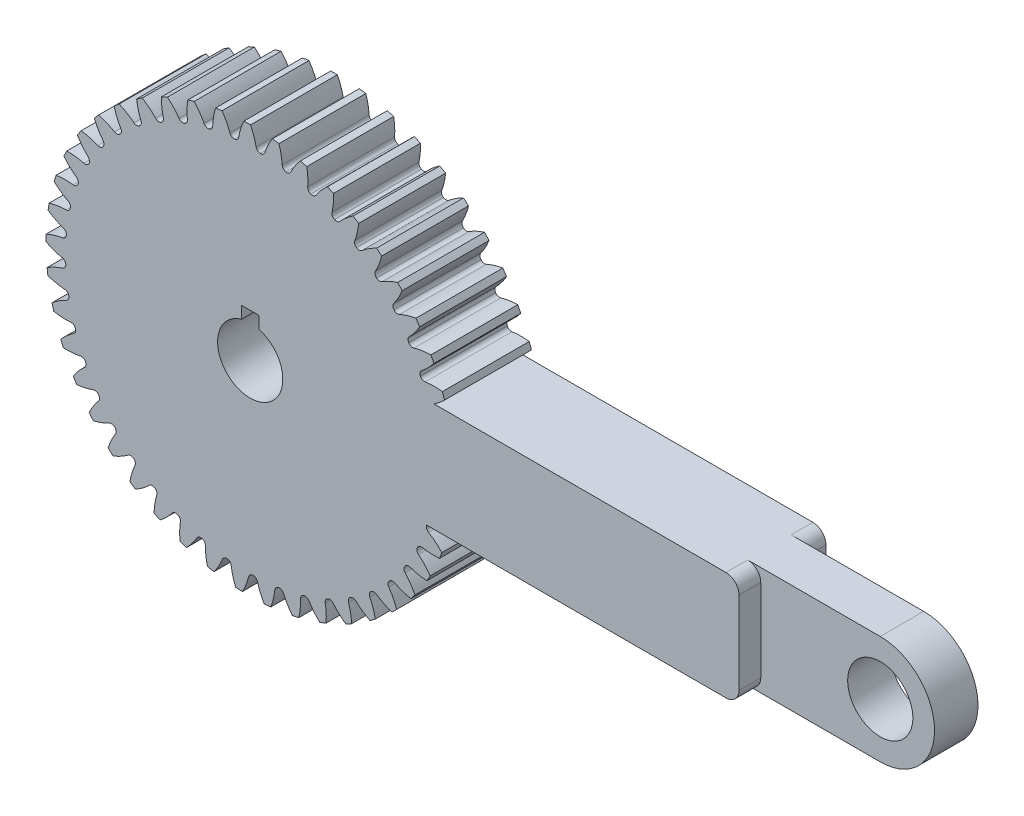
from build123d import *

# Parameters (mm, degrees)
SKETCH1_R           = 7.5
BOSS_EXTRUDE1_DEPTH = 20
SKETCH2_W           = 40
SKETCH2_H           = 7.746884482
SKETCH2_H_2         = 5
CUT_EXTRUDE1_DEPTH  = 41
FILLET1_R           = 3
SCALE1_SCALE        = 0.3


with BuildPart() as part:
    # Sketch1 → Boss-Extrude1 (new body)
    with BuildSketch(Plane(origin=(0, 0, 0), x_dir=(-1, 0, 0), z_dir=(0, 0, -1))):
        with BuildLine():
            Line((-140, -12.5), (-40.620192023, -12.5))
            ThreePointArc((-40.620192023, -12.5), (-40.610112054, -12.532709162), (-40.600005747, -12.565410195))
            ThreePointArc((-40.600005747, -12.565410195), (-40.621924881, -13.219969243), (-41.044194735, -13.720585031))
            ThreePointArc((-41.044194735, -13.720585031), (-42.659259377, -14.876128654), (-44.106676084, -16.235797635))
            ThreePointArc((-44.106676084, -16.235797635), (-43.835198922, -16.955097625), (-43.551992177, -17.669860707))
            ThreePointArc((-43.551992177, -17.669860707), (-41.566460224, -17.699832016), (-39.594088642, -17.469645664))
            ThreePointArc((-39.594088642, -17.469645664), (-38.94485587, -17.555812971), (-38.488181859, -18.025256092))
            ThreePointArc((-38.488181859, -18.025256092), (-38.472167175, -18.059411753), (-38.45612218, -18.093553185))
            ThreePointArc((-38.45612218, -18.093553185), (-38.386730986, -18.744792664), (-38.735219087, -19.299305098))
            ThreePointArc((-38.735219087, -19.299305098), (-40.173745442, -20.668376604), (-41.417846641, -22.216254852))
            ThreePointArc((-41.417846641, -22.216254852), (-41.048904266, -22.890772346), (-40.668977875, -23.559164642))
            ThreePointArc((-40.668977875, -23.559164642), (-38.698597783, -23.312511632), (-36.777456933, -22.81006437))
            ThreePointArc((-36.777456933, -22.81006437), (-36.122550279, -22.805037364), (-35.604986733, -23.206355158))
            ThreePointArc((-35.604986733, -23.206355158), (-35.584374354, -23.237949606), (-35.563733938, -23.269525744))
            ThreePointArc((-35.563733938, -23.269525744), (-35.404383037, -23.904770017), (-35.672306461, -24.502386144))
            ThreePointArc((-35.672306461, -24.502386144), (-36.906295249, -26.058338114), (-37.922865925, -27.764297939))
            ThreePointArc((-37.922865925, -27.764297939), (-37.463639381, -28.38090422), (-36.994388179, -28.989916235))
            ThreePointArc((-36.994388179, -28.989916235), (-35.077511154, -28.471439728), (-33.244993859, -27.706511118))
            ThreePointArc((-33.244993859, -27.706511118), (-32.597160335, -27.610387645), (-32.02878104, -27.935768919))
            ThreePointArc((-32.02878104, -27.935768919), (-32.003972162, -27.964187202), (-31.979138069, -27.992583453))
            ThreePointArc((-31.979138069, -27.992583453), (-31.732929044, -28.599468214), (-31.915072966, -29.228556115))
            ThreePointArc((-31.915072966, -29.228556115), (-32.920506, -30.941103714), (-33.68975976, -32.771940549))
            ThreePointArc((-33.68975976, -32.771940549), (-33.149187369, -33.318634077), (-32.599744797, -33.856412084))
            ThreePointArc((-32.599744797, -33.856412084), (-30.773680671, -33.076203635), (-29.065454795, -32.063682143))
            ThreePointArc((-29.065454795, -32.063682143), (-28.437303745, -31.878333137), (-27.829171557, -32.121444713))
            ThreePointArc((-27.829171557, -32.121444713), (-27.800649056, -32.146133703), (-27.772104652, -32.170797366))
            ThreePointArc((-27.772104652, -32.170797366), (-27.443829683, -32.737510293), (-27.536648879, -33.385825488))
            ThreePointArc((-27.536648879, -33.385825488), (-28.293956547, -35.221635925), (-28.800920743, -37.141714612))
            ThreePointArc((-28.800920743, -37.141714612), (-28.189524132, -37.607854621), (-27.570584464, -38.063931383))
            ThreePointArc((-27.570584464, -38.063931383), (-25.870875498, -37.037176862), (-24.320189715, -35.796770067))
            ThreePointArc((-24.320189715, -35.796770067), (-23.723947383, -35.525803135), (-23.087898904, -35.681913124))
            ThreePointArc((-23.087898904, -35.681913124), (-23.056217939, -35.702392278), (-23.024518809, -35.722843303))
            ThreePointArc((-23.024518809, -35.722843303), (-22.620567394, -36.238353972), (-22.622255243, -36.893277744))
            ThreePointArc((-22.622255243, -36.893277744), (-23.116697415, -38.816619056), (-23.351504565, -40.788567449))
            ThreePointArc((-23.351504565, -40.788567449), (-22.681183873, -41.165081053), (-22.004794066, -41.530579554))
            ThreePointArc((-22.004794066, -41.530579554), (-20.464523162, -40.27726357), (-19.101559806, -38.83311458))
            ThreePointArc((-19.101559806, -38.83311458), (-18.548831372, -38.481803785), (-17.897246562, -38.547873684))
            ThreePointArc((-17.897246562, -38.547873684), (-17.863023766, -38.563744397), (-17.828786897, -38.579584728))
            ThreePointArc((-17.828786897, -38.579584728), (-17.357021491, -39.033859312), (-17.267545142, -39.682644314))
            ThreePointArc((-17.267545142, -39.682644314), (-17.489498062, -41.656080851), (-17.447577912, -43.641517217))
            ThreePointArc((-17.447577912, -43.641517217), (-16.731380169, -43.921076007), (-16.010705382, -44.188882235))
            ThreePointArc((-16.010705382, -44.188882235), (-14.65985216, -42.733399158), (-13.511139763, -41.11361669))
            ThreePointArc((-13.511139763, -41.11361669), (-13.012683457, -40.688799898), (-12.358244672, -40.663543729))
            ThreePointArc((-12.358244672, -40.663543729), (-12.322146155, -40.674497098), (-12.286037928, -40.68541842))
            ThreePointArc((-12.286037928, -40.68541842), (-11.755640908, -41.069614981), (-11.576741916, -41.699633351))
            ThreePointArc((-11.576741916, -41.699633351), (-11.521885523, -43.684754415), (-11.204054002, -45.645034494))
            ThreePointArc((-11.204054002, -45.645034494), (-10.455919182, -45.822197176), (-9.704986529, -45.987098587))
            ThreePointArc((-9.704986529, -45.987098587), (-8.569843811, -44.35777774), (-7.657740753, -42.593889017))
            ThreePointArc((-7.657740753, -42.593889017), (-7.22325846, -42.103834802), (-6.578703608, -41.98774415))
            ThreePointArc((-6.578703608, -41.98774415), (-6.541431984, -41.993566979), (-6.504155206, -41.999356722))
            ThreePointArc((-6.504155206, -41.999356722), (-5.925450147, -42.30599731), (-5.660610577, -42.904986457))
            ThreePointArc((-5.660610577, -42.904986457), (-5.330012588, -44.863153925), (-4.742455924, -46.760123094))
            ThreePointArc((-4.742455924, -46.760123094), (-3.976945621, -46.831441399), (-3.210371153, -46.890228375))
            ThreePointArc((-3.210371153, -46.890228375), (-2.3130332, -45.118782634), (-1.65529253, -43.245119744))
            ThreePointArc((-1.65529253, -43.245119744), (-1.293240953, -42.699366455), (-0.671115561, -42.494700892))
            ThreePointArc((-0.671115561, -42.494700892), (-0.633396281, -42.495279846), (-0.595676502, -42.495825319))
            ThreePointArc((-0.595676502, -42.495825319), (0.020072761, -42.718941524), (0.365698108, -43.275242806))
            ThreePointArc((0.365698108, -43.275242806), (0.965602978, -45.168343175), (1.811448663, -46.965079088))
            ThreePointArc((1.811448663, -46.965079088), (2.579434662, -46.929164885), (3.346730446, -46.880693204))
            ThreePointArc((3.346730446, -46.880693204), (3.98879797, -45.001601746), (4.379374079, -43.054633405))
            ThreePointArc((4.379374079, -43.054633405), (4.661948018, -42.46380351), (5.249534987, -42.174546618))
            ThreePointArc((5.249534987, -42.174546618), (5.28696776, -42.169870428), (5.324396368, -42.165161014))
            ThreePointArc((5.324396368, -42.165161014), (5.965204976, -42.300410133), (6.384888895, -42.803195778))
            ThreePointArc((6.384888895, -42.803195778), (7.242424181, -44.594382004), (8.330095463, -46.255913239))
            ThreePointArc((8.330095463, -46.255913239), (9.085609184, -46.113465558), (9.838691744, -45.958678666))
            ThreePointArc((9.838691744, -45.958678666), (10.212991726, -44.008515868), (10.328801154, -42.026137602))
            ThreePointArc((10.328801154, -42.026137602), (10.526397473, -41.401730931), (11.068009308, -41.033512767))
            ThreePointArc((11.068009308, -41.033512767), (11.104426988, -41.02367245), (11.14083592, -41.013799812))
            ThreePointArc((11.14083592, -41.013799812), (11.794231262, -41.058549375), (12.279805082, -41.498033232))
            ThreePointArc((12.279805082, -41.498033232), (13.378279836, -43.152441912), (14.68660643, -44.646428654))
            ThreePointArc((14.68660643, -44.646428654), (15.414942657, -44.400220077), (16.139154098, -44.142130726))
            ThreePointArc((16.139154098, -44.142130726), (16.238401215, -42.158854289), (16.077189862, -40.179650834))
            ThreePointArc((16.077189862, -40.179650834), (16.185962575, -39.533820753), (16.671057417, -39.093808264))
            ThreePointArc((16.671057417, -39.093808264), (16.705751176, -39.078995351), (16.740431772, -39.064151649))
            ThreePointArc((16.740431772, -39.064151649), (17.393696251, -39.017530657), (17.935708832, -39.385158673))
            ThreePointArc((17.935708832, -39.385158673), (19.253742491, -40.870588623), (20.757259308, -42.16795212))
            ThreePointArc((20.757259308, -42.16795212), (21.444241806, -41.822774816), (22.125486176, -41.466406421))
            ThreePointArc((22.125486176, -41.466406421), (21.947748694, -39.488618565), (21.512654358, -37.551112866))
            ThreePointArc((21.512654358, -37.551112866), (21.530486327, -36.896429724), (21.949622357, -36.393187253))
            ThreePointArc((21.949622357, -36.393187253), (21.981916919, -36.37369006), (22.014194163, -36.35416421))
            ThreePointArc((22.014194163, -36.35416421), (22.654612728, -36.217080086), (23.242514411, -36.5056968))
            ThreePointArc((23.242514411, -36.5056968), (24.754452949, -37.793235816), (26.423895745, -38.868724364))
            ThreePointArc((26.423895745, -38.868724364), (27.056153181, -38.431296817), (27.681170833, -37.983585683))
            ThreePointArc((27.681170833, -37.983585683), (27.229908211, -36.049781799), (26.529399506, -34.1916852))
            ThreePointArc((26.529399506, -34.1916852), (26.455943653, -33.540891659), (26.800962865, -32.984214248))
            ThreePointArc((26.800962865, -32.984214248), (26.830229654, -32.960412266), (26.859475304, -32.936584316))
            ThreePointArc((26.859475304, -32.936584316), (27.474582938, -32.711705248), (28.096930885, -32.915693064))
            ThreePointArc((28.096930885, -32.915693064), (29.773346139, -33.980280664), (31.576221108, -34.8129611))
            ThreePointArc((31.576221108, -34.8129611), (32.14144731, -34.29179734), (32.698072986, -33.761457655))
            ThreePointArc((32.698072986, -33.761457655), (31.982068538, -31.909277036), (31.029780071, -30.166755274))
            ThreePointArc((31.029780071, -30.166755274), (30.866466129, -29.53251829), (31.130653116, -28.933241031))
            ThreePointArc((31.130653116, -28.933241031), (31.156322487, -28.905597539), (31.181967311, -28.877931273))
            ThreePointArc((31.181967311, -28.877931273), (31.759791642, -28.569634276), (32.404472559, -28.685022803))
            ThreePointArc((32.404472559, -28.685022803), (34.212735012, -29.505938), (36.113951245, -30.079603147))
            ThreePointArc((36.113951245, -30.079603147), (36.601144728, -29.484847034), (37.078544342, -28.882201257))
            ThreePointArc((37.078544342, -28.882201257), (36.11173428, -27.147694492), (34.926201261, -25.554663771))
            ThreePointArc((34.926201261, -25.554663771), (34.676207952, -24.949328045), (34.854420615, -24.31911519))
            ThreePointArc((34.854420615, -24.31911519), (34.875992943, -24.288168236), (34.897537793, -24.257202146))
            ThreePointArc((34.897537793, -24.257202146), (35.426832129, -23.871487871), (36.081298034, -23.896031202))
            ThreePointArc((36.081298034, -23.896031202), (37.986211915, -24.457295816), (39.948764399, -24.760779934))
            ThreePointArc((39.948764399, -24.760779934), (40.348442496, -24.104007719), (40.737324009, -23.440785665))
            ThreePointArc((40.737324009, -23.440785665), (39.538526191, -21.857712954), (38.142823673, -20.445179806))
            ThreePointArc((38.142823673, -20.445179806), (37.811016831, -19.880527509), (37.899786463, -19.231645433))
            ThreePointArc((37.899786463, -19.231645433), (37.916841867, -19.197997365), (37.933867398, -19.164334172))
            ThreePointArc((37.933867398, -19.164334172), (38.404329625, -18.708710107), (39.055842085, -18.641930535))
            ThreePointArc((39.055842085, -18.641930535), (41.020330412, -18.932620188), (43.006020296, -18.960016305))
            ThreePointArc((43.006020296, -18.960016305), (43.310403727, -18.254011312), (43.603198002, -17.543121843))
            ThreePointArc((43.603198002, -17.543121843), (42.195745664, -16.142295897), (40.617039408, -14.937753671))
            ThreePointArc((40.617039408, -14.937753671), (40.209877277, -14.424775119), (40.207476078, -13.769853574))
            ThreePointArc((40.207476078, -13.769853574), (40.219682594, -13.734159313), (40.231857422, -13.698454232))
            ThreePointArc((40.231857422, -13.698454232), (40.63433053, -13.181788582), (41.270208595, -13.024985895))
            ThreePointArc((41.270208595, -13.024985895), (43.256034837, -13.039442644), (45.226212926, -12.790217525))
            ThreePointArc((45.226212926, -12.790217525), (45.429377215, -12.048721338), (45.620385344, -11.304001109))
            ThreePointArc((45.620385344, -11.304001109), (44.031672944, -10.112687412), (42.300690672, -9.139581153))
            ThreePointArc((42.300690672, -9.139581153), (41.826098199, -8.68826089), (41.732572906, -8.040047178))
            ThreePointArc((41.732572906, -8.040047178), (41.739692948, -8.003001473), (41.746780105, -7.965949462))
            ThreePointArc((41.746780105, -7.965949462), (42.073430412, -7.398298536), (42.681297439, -7.15452472))
            ThreePointArc((42.681297439, -7.15452472), (44.649809747, -6.892467181), (46.566128766, -6.37147171))
            ThreePointArc((46.566128766, -6.37147171), (46.66411955, -5.608916708), (46.749623777, -4.844860852))
            ThreePointArc((46.749623777, -4.844860852), (45.010573796, -3.886246969), (43.161007109, -3.163517084))
            ThreePointArc((43.161007109, -3.163517084), (42.628221696, -2.782639544), (42.445392673, -2.153750409))
            ThreePointArc((42.445392673, -2.153750409), (42.447287658, -2.116074312), (42.4491492, -2.078396547))
            ThreePointArc((42.4491492, -2.078396547), (42.693618828, -1.470809025), (43.261643377, -1.144808859))
            ThreePointArc((43.261643377, -1.144808859), (45.174526899, -0.611337685), (46.999687877, 0.171287555))
            ThreePointArc((46.999687877, 0.171287555), (46.990597877, 0.940059105), (46.968933961, 1.70857911))
            ThreePointArc((46.968933961, 1.70857911), (45.113395028, 2.415834851), (43.181243637, 2.874121247))
            ThreePointArc((43.181243637, 2.874121247), (42.600635347, 3.177142714), (42.332061153, 3.774466662))
            ThreePointArc((42.332061153, 3.774466662), (42.328694196, 3.812039829), (42.32529389, 3.849609992))
            ThreePointArc((42.32529389, 3.849609992), (42.482824517, 4.485308111), (42.999950636, 4.887189403))
            ThreePointArc((42.999950636, 4.887189403), (44.81997327, 5.681690805), (46.518451526, 6.710712902))
            ThreePointArc((46.518451526, 6.710712902), (46.402457668, 7.470737737), (46.274047271, 8.228763524))
            ThreePointArc((46.274047271, 8.228763524), (44.338135341, 8.670895193), (42.361006376, 8.855818076))
            ThreePointArc((42.361006376, 8.855818076), (41.743876089, 9.075085504), (41.394784214, 9.629218032))
            ThreePointArc((41.394784214, 9.629218032), (41.38622085, 9.66595695), (41.37762488, 9.702688252))
            ThreePointArc((41.37762488, 9.702688252), (41.445150351, 10.354123826), (41.901312769, 10.824064083))
            ThreePointArc((41.901312769, 10.824064083), (43.593049843, 11.864131645), (45.131786429, 13.119521856))
            ThreePointArc((45.131786429, 13.119521856), (44.911146403, 13.856006957), (44.678488887, 14.588784416))
            ThreePointArc((44.678488887, 14.588784416), (42.699884283, 14.757186423), (40.716260311, 14.665146481))
            ThreePointArc((40.716260311, 14.665146481), (40.074619765, 14.796392077), (39.651804886, 15.296547627))
            ThreePointArc((39.651804886, 15.296547627), (39.638211791, 15.331737214), (39.624587467, 15.366914722))
            ThreePointArc((39.624587467, 15.366914722), (39.600793476, 16.021408299), (39.98711351, 16.550260668))
            ThreePointArc((39.98711351, 16.550260668), (41.517637287, 17.815650659), (42.866682446, 19.27297424))
            ThreePointArc((42.866682446, 19.27297424), (42.545690758, 19.971584762), (42.213314538, 20.664851213))
            ThreePointArc((42.213314538, 20.664851213), (40.230528549, 20.556245806), (38.279018553, 20.18903449))
            ThreePointArc((38.279018553, 20.18903449), (37.625356552, 20.229703709), (37.137048279, 20.666147321))
            ThreePointArc((37.137048279, 20.666147321), (37.118690028, 20.699102653), (37.100302532, 20.732041676))
            ThreePointArc((37.100302532, 20.732041676), (36.985652202, 21.376854283), (37.294610571, 21.954325254))
            ThreePointArc((37.294610571, 21.954325254), (38.634131147, 23.420408297), (39.767227249, 25.051300104))
            ThreePointArc((39.767227249, 25.051300104), (39.352131638, 25.698438387), (38.926506039, 26.338700188))
            ThreePointArc((38.926506039, 26.338700188), (36.978131338, 25.955201246), (35.09671924, 25.319965908))
            ThreePointArc((35.09671924, 25.319965908), (34.443758572, 25.269267169), (33.899461271, 25.633503966))
            ThreePointArc((33.899461271, 25.633503966), (33.876695185, 25.663583603), (33.853902408, 25.693643022))
            ThreePointArc((33.853902408, 25.693643022), (33.650627278, 26.316224115), (33.876210459, 26.931073872))
            ThreePointArc((33.876210459, 26.931073872), (34.99865559, 28.569314328), (35.893748209, 30.342030906))
            ThreePointArc((35.893748209, 30.342030906), (35.392628038, 30.925101141), (34.882037378, 31.499896323))
            ThreePointArc((34.882037378, 31.499896323), (33.005996862, 30.848968218), (31.231302209, 29.958072991))
            ThreePointArc((31.231302209, 29.958072991), (30.59175201, 29.816993087), (30.002059808, 30.101933613))
            ThreePointArc((30.002059808, 30.101933613), (29.975329004, 30.128552091), (29.948574583, 30.155146832))
            ThreePointArc((29.948574583, 30.155146832), (29.66063117, 30.743378578), (29.798448445, 31.383639771))
            ThreePointArc((29.798448445, 31.383639771), (30.681971013, 33.162151153), (31.321638188, 35.042188591))
            ThreePointArc((31.321638188, 35.042188591), (30.744247192, 35.549841978), (30.158629536, 36.047982807))
            ThreePointArc((30.158629536, 36.047982807), (28.391438201, 35.142295113), (26.758003406, 34.013080259))
            ThreePointArc((26.758003406, 34.013080259), (26.144311793, 33.784365151), (25.520702379, 33.984463363))
            ThreePointArc((25.520702379, 33.984463363), (25.490527141, 34.007102583), (25.460331819, 34.02971501))
            ThreePointArc((25.460331819, 34.02971501), (25.093324616, 34.572148148), (25.140693527, 35.22535882))
            ThreePointArc((25.140693527, 35.22535882), (25.76809677, 37.109524427), (26.139888108, 39.060289934))
            ThreePointArc((26.139888108, 39.060289934), (25.497464545, 39.482645577), (24.848218276, 39.89443631))
            ThreePointArc((24.848218276, 39.89443631), (23.22427249, 38.751617208), (21.763890504, 37.40606161))
            ThreePointArc((21.763890504, 37.40606161), (21.188002286, 37.094162977), (20.542613507, 37.205524191))
            ThreePointArc((20.542613507, 37.205524191), (20.509581162, 37.223743506), (20.476532658, 37.241933493))
            ThreePointArc((20.476532658, 37.241933493), (20.037605041, 37.728010179), (19.993603606, 38.381456328))
            ThreePointArc((19.993603606, 38.381456328), (20.352675833, 40.334603019), (20.449354839, 42.318127164))
            ThreePointArc((20.449354839, 42.318127164), (19.754402753, 42.646964392), (19.054164712, 42.964389989))
            ThreePointArc((19.054164712, 42.964389989), (17.605072733, 41.606683153), (16.346168228, 40.07097652))
            ThreePointArc((16.346168228, 40.07097652), (15.819292415, 39.681965114), (15.16468603, 39.70242181))
            ThreePointArc((15.16468603, 39.70242181), (15.129439515, 39.715866602), (15.094181079, 39.729280104))
            ThreePointArc((15.094181079, 39.729280104), (14.591876277, 40.149539406), (14.457360934, 40.790502446))
            ThreePointArc((14.457360934, 40.790502446), (14.541113213, 42.774614444), (14.360798139, 44.752290185))
            ThreePointArc((14.360798139, 44.752290185), (13.626843983, 44.981208555), (12.889243505, 45.198090688))
            ThreePointArc((12.889243505, 45.198090688), (11.64321026, 43.651922338), (10.610286382, 41.955955452))
            ThreePointArc((10.610286382, 41.955955452), (10.142678012, 41.497402938), (9.491595189, 41.42655695))
            ThreePointArc((9.491595189, 41.42655695), (9.454820537, 41.434965532), (9.418038436, 41.443341468))
            ThreePointArc((9.418038436, 41.443341468), (8.862133239, 41.789603519), (8.639722176, 42.405607833))
            ThreePointArc((8.639722176, 42.405607833), (8.446524364, 44.382066654), (7.992724839, 46.315400783))
            ThreePointArc((7.992724839, 46.315400783), (7.234054194, 46.439944659), (6.473447835, 46.552061964))
            ThreePointArc((6.473447835, 46.552061964), (5.454725944, 44.847526507), (4.66788738, 43.024309436))
            ThreePointArc((4.66788738, 43.024309436), (4.268647918, 42.505141016), (3.633761244, 42.344371281))
            ThreePointArc((3.633761244, 42.344371281), (3.596174232, 42.347579989), (3.558584387, 42.350755332))
            ThreePointArc((3.558584387, 42.350755332), (2.959898858, 42.616280534), (2.653921053, 43.1953363))
            ThreePointArc((2.653921053, 43.1953363), (2.187533527, 45.12567242), (1.469082241, 46.977034787))
            ThreePointArc((1.469082241, 46.977034787), (0.700461769, 46.994780064), (-0.068346134, 46.999950306))
            ThreePointArc((-0.068346134, 46.999950306), (-0.839928408, 45.170224587), (-1.36536674, 43.255244175))
            ThreePointArc((-1.36536674, 43.255244175), (-1.688466552, 42.685564873), (-2.29479973, 42.438000591))
            ThreePointArc((-2.29479973, 42.438000591), (-2.332467513, 42.435946971), (-2.370133459, 42.433859916))
            ThreePointArc((-2.370133459, 42.433859916), (-2.999946588, 42.613480124), (-3.383535624, 43.144316679))
            ThreePointArc((-3.383535624, 43.144316679), (-4.114035163, 44.990958303), (-5.083154371, 46.724314245))
            ThreePointArc((-5.083154371, 46.724314245), (-5.846764347, 46.634915532), (-6.608809824, 46.533038077))
            ThreePointArc((-6.608809824, 46.533038077), (-7.11823451, 44.613735625), (-7.372045549, 42.644264789))
            ThreePointArc((-7.372045549, 42.644264789), (-7.612716941, 42.035162764), (-8.178695037, 41.705622492))
            ThreePointArc((-8.178695037, 41.705622492), (-8.215710432, 41.698346515), (-8.252719354, 41.691037685))
            ThreePointArc((-8.252719354, 41.691037685), (-8.901401486, 41.781256796), (-9.355135629, 42.25354201))
            ThreePointArc((-9.355135629, 42.25354201), (-10.335528838, 43.980546358), (-11.536453166, 45.562158074))
            ThreePointArc((-11.536453166, 45.562158074), (-12.280189846, 45.367355415), (-13.020640547, 45.160413193))
            ThreePointArc((-13.020640547, 45.160413193), (-13.257992273, 43.188891047), (-13.235235877, 41.203263296))
            ThreePointArc((-13.235235877, 41.203263296), (-13.388794454, 40.566594026), (-13.903401349, 40.161491891))
            ThreePointArc((-13.903401349, 40.161491891), (-13.939043892, 40.149135176), (-13.974675453, 40.136746829))
            ThreePointArc((-13.974675453, 40.136746829), (-14.629600729, 40.135808829), (-15.14464856, 40.540350208))
            ThreePointArc((-15.14464856, 40.540350208), (-16.3558532, 42.114103106), (-17.765208023, 43.513186322))
            ThreePointArc((-17.765208023, 43.513186322), (-18.474595418, 43.21677133), (-19.179039313, 42.908792235))
            ThreePointArc((-19.179039313, 42.908792235), (-19.139698298, 40.923423831), (-18.840817394, 38.960287151))
            ThreePointArc((-18.840817394, 38.960287151), (-18.904274313, 38.30844268), (-19.357493769, 37.835663533))
            ThreePointArc((-19.357493769, 37.835663533), (-19.391069719, 37.818466589), (-19.424630391, 37.80123985))
            ThreePointArc((-19.424630391, 37.80123985), (-20.073051434, 37.709162997), (-20.639388134, 38.038086604))
            ThreePointArc((-20.639388134, 38.038086604), (-22.057829484, 39.427956741), (-23.648183313, 40.617279894))
            ThreePointArc((-23.648183313, 40.617279894), (-24.309414005, 40.225021949), (-24.964139895, 39.822000444))
            ThreePointArc((-24.964139895, 39.822000444), (-24.648871866, 37.861428719), (-24.079683832, 35.958993334))
            ThreePointArc((-24.079683832, 35.958993334), (-24.051803976, 35.304661071), (-24.434814591, 34.773407022))
            ThreePointArc((-24.434814591, 34.773407022), (-24.46567043, 34.751704569), (-24.496506993, 34.729974736))
            ThreePointArc((-24.496506993, 34.729974736), (-25.125803026, 34.548551201), (-25.732405494, 34.795454911))
            ThreePointArc((-25.732405494, 34.795454911), (-27.330475208, 35.974390046), (-29.070873614, 36.930804315))
            ThreePointArc((-29.070873614, 36.930804315), (-29.671077499, 36.450338271), (-30.263341889, 35.960118711))
            ThreePointArc((-30.263341889, 35.960118711), (-29.678283181, 34.062503965), (-28.849866614, 32.257798613))
            ThreePointArc((-28.849866614, 32.257798613), (-28.731192632, 31.613714394), (-29.036539541, 31.034325697))
            ThreePointArc((-29.036539541, 31.034325697), (-29.064074696, 31.008540148), (-29.091586951, 30.982730168))
            ThreePointArc((-29.091586951, 30.982730168), (-29.689509443, 30.715491155), (-30.324570852, 30.875569268))
            ThreePointArc((-30.324570852, 30.875569268), (-32.07116432, 31.82062277), (-33.927732427, 32.525512638))
            ThreePointArc((-33.927732427, 32.525512638), (-34.455227221, 31.96619022), (-34.973502358, 31.398314171))
            ThreePointArc((-34.973502358, 31.398314171), (-34.130040473, 29.600591317), (-33.058519558, 27.928742536))
            ThreePointArc((-33.058519558, 27.928742536), (-32.851361306, 27.307442725), (-33.073101278, 26.691196524))
            ThreePointArc((-33.073101278, 26.691196524), (-33.096779807, 26.661829765), (-33.120432261, 26.632442))
            ThreePointArc((-33.120432261, 26.632442), (-33.675343329, 26.284589011), (-34.326502932, 26.35472579))
            ThreePointArc((-34.326502932, 26.35472579), (-36.187624699, 27.047503267), (-38.124226522, 27.487148854))
            ThreePointArc((-38.124226522, 27.487148854), (-38.568745137, 26.859856637), (-39.002943386, 26.225377162))
            ThreePointArc((-39.002943386, 26.225377162), (-37.917495349, 24.562536828), (-36.623726023, 23.056085253))
            ThreePointArc((-36.623726023, 23.056085253), (-36.332115599, 22.469662746), (-36.465932718, 21.828553571))
            ThreePointArc((-36.465932718, 21.828553571), (-36.485293747, 21.796177193), (-36.50462603, 21.763783642))
            ThreePointArc((-36.50462603, 21.763783642), (-37.005724963, 21.342087241), (-37.660308679, 21.320917552))
            ThreePointArc((-37.660308679, 21.320917552), (-39.599734126, 21.747934878), (-41.578675913, 21.913778984))
            ThreePointArc((-41.578675913, 21.913778984), (-41.9315663, 21.230726498), (-42.273236485, 20.541993016))
            ThreePointArc((-42.273236485, 20.541993016), (-40.966929308, 19.0464005), (-39.47609332, 17.734667497))
            ThreePointArc((-39.47609332, 17.734667497), (-39.10570659, 17.194536341), (-39.148996258, 16.541042652))
            ThreePointArc((-39.148996258, 16.541042652), (-39.163662945, 16.506286824), (-39.178298777, 16.471517992))
            ThreePointArc((-39.178298777, 16.471517992), (-39.615832254, 15.984186018), (-40.261099354, 15.872121906))
            ThreePointArc((-40.261099354, 15.872121906), (-42.241079772, 16.025067676), (-44.223843672, 15.913882333))
            ThreePointArc((-44.223843672, 15.913882333), (-44.478237222, 15.188364417), (-44.720729121, 14.458782343))
            ThreePointArc((-44.720729121, 14.458782343), (-43.548810179, 13.42223114), (-42.284958081, 12.5))
            Line((-42.284958081, 12.5), (-140, 12.5))
            ThreePointArc((-140, 12.5), (-152.5, 0), (-140, -12.5))
        make_face()
        with Locations(Location((-140, 0, 0), (0, 0, 180))):
            Circle(SKETCH1_R, mode=Mode.SUBTRACT)
        with BuildLine():
            Line((-2, 7.228416147), (-2, 10))
            Line((-2, 10), (2, 10))
            Line((2, 10), (2, 7.228416147))
            ThreePointArc((2, 7.228416147), (0, -7.5), (-2, 7.228416147))
        make_face(mode=Mode.SUBTRACT)
    extrude(amount=-BOSS_EXTRUDE1_DEPTH)

    # Sketch2 → Cut-Extrude1 (cut)
    with BuildSketch(Plane.XZ.offset(12.5)):
        with Locations((132.5, 18.873442241)):
            Rectangle(SKETCH2_W, SKETCH2_H)
        with Locations((132.5, 2.5)):
            Rectangle(SKETCH2_W, SKETCH2_H_2)
    extrude(amount=-CUT_EXTRUDE1_DEPTH, mode=Mode.SUBTRACT)

    # Fillet1
    fillet1_edges = [part.edges().sort_by_distance(p)[0] for p in [
        (112.5, 12.5, 17.5),
        (112.5, -12.5, 17.5),
        (112.5, 12.5, 2.5),
        (112.5, -12.5, 2.5),
    ]]
    fillet(fillet1_edges, radius=FILLET1_R)


with BuildPart() as part_1:
    # Scale1: scaled about (0, 0, 0)
    add(part.part.scale(SCALE1_SCALE))


solid = part_1.part
